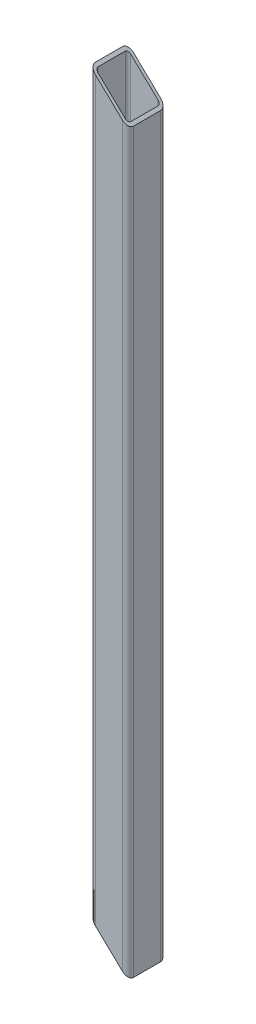
SolidWorks part; units mm, degrees
material "Q235B"
ref_plane "Front Plane" through (0, 0, 0) normal (0, 0, 1) x (1, 0, 0)
ref_plane "Top Plane" through (0, 0, 0) normal (0, 1, 0) x (1, 0, 0)
ref_plane "Right Plane" through (0, 0, 0) normal (1, 0, 0) x (0, 0, -1)
sketch "feature 17 (ProfileFeature) (+16 more in 12 files) Sketch1" plane through (0, 0, 0) normal (0, 0, 1) x (1, 0, 0)
  line L0 (0, 0) -> (0, 1420.5)
  dimension "D1" = 1420.5
other "feature 19 (WeldMemberFeat) (+4 more in 5 files) Cold-formed Hollow Structural Square Steel(gb t6728-2002) 70×70×5(1)"
ref_plane "Plane1" through (0, 0, 0) normal (0, 1, 0) x (-1, 0, 0)
sketch "Sketch1" plane through (0, 0, 0) normal (0, 1, 0) x (-1, 0, 0)
  line L0 (-25, -30) -> (25, -30)
  line L1 (-30, -25) -> (-30, 25)
  line L2 (25, 30) -> (-25, 30)
  line L3 (30, 25) -> (30, -25)
  line L4 (-25, -35) -> (25, -35)
  line L5 (-35, -25) -> (-35, 25)
  line L6 (25, 35) -> (-25, 35)
  line L7 (35, 25) -> (35, -25)
  arc A0 (35, 25) -> (25, 35) centre (25, 25) ccw
  arc A1 (25, -35) -> (35, -25) centre (25, -25) ccw
  arc A2 (-35, -25) -> (-25, -35) centre (-25, -25) ccw
  arc A3 (-25, 35) -> (-35, 25) centre (-25, 25) ccw
  arc A4 (-25, 30) -> (-30, 25) centre (-25, 25) ccw
  arc A5 (30, 25) -> (25, 30) centre (25, 25) ccw
  arc A6 (25, -30) -> (30, -25) centre (25, -25) ccw
  arc A7 (-30, -25) -> (-25, -30) centre (-25, -25) ccw
  point P0 (-35, 0)
  point P1 (35, 0)
  point P2 (0, 35)
  point P3 (0, -35)
  point P4 (0, 0)
  point P5 (-35, -35)
  point P6 (35, -35)
  point P7 (35, 35)
  point P8 (-35, 35)
  point P33 (0, 0)
  dimension "D1" = 10
  dimension "D2" = 70
  dimension "D3" = 5
sketch "0:feat:20/0 feature 20/0 (ProfileFeature) (+11 more in 7 files) Sketch2" plane through (0, 0, 35) normal (0, 0, 1) x (1, 0, 0)
  line L1 (-35, 1420.5) -> (-35, 0) construction
  line L4 (-35, 66.7136) -> (35, 0)
  line L5 (35, 0) -> (-35, 0)
  line L6 (-35, 0) -> (-35, 66.7136)
  line L7 (-35, 1420.5) -> (35, 1353.7864)
  line L8 (35, 1420.5) -> (35, 0) construction
  line L9 (35, 1353.7864) -> (35, 1420.5)
  line L10 (35, 1420.5) -> (-35, 1420.5)
  dimension "D1" = 980
extrude "Cut-Extrude1" cut sketch "0:feat:20/0 feature 20/0 (ProfileFeature) (+11 more in 7 files) Sketch2" against normal through all both and the other way through all
